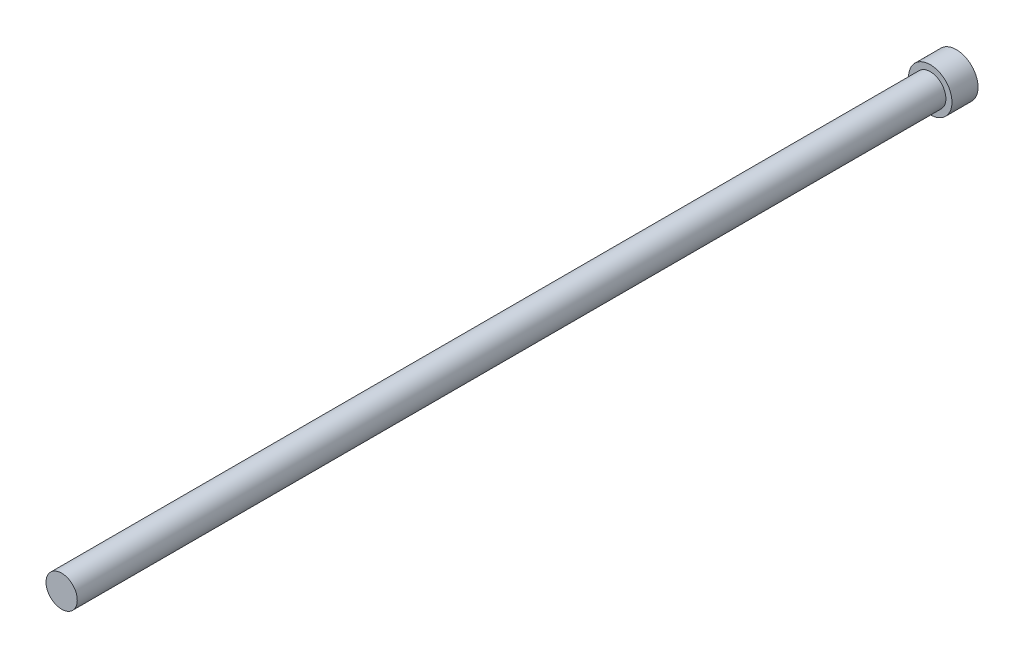
from build123d import *

# Parameters (mm, degrees)
SKETCH1_R           = 9
BOSS_EXTRUDE1_DEPTH = 500
SKETCH2_R           = 12.5
BOSS_EXTRUDE2_DEPTH = 15


with BuildPart() as part:
    # Sketch1 → Boss-Extrude1 (new body)
    with BuildSketch(Plane.XY):
        Circle(SKETCH1_R)
    extrude(amount=BOSS_EXTRUDE1_DEPTH)

    # Sketch2 → Boss-Extrude2 (add)
    with BuildSketch(Plane(origin=(0, 0, 0), x_dir=(-1, 0, 0), z_dir=(0, 0, -1))):
        Circle(SKETCH2_R)
    extrude(amount=BOSS_EXTRUDE2_DEPTH)


solid = part.part
